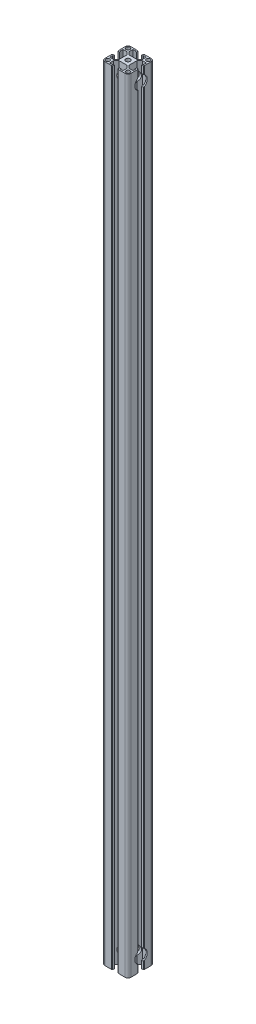
from build123d import *

# Parameters (mm, degrees)
SKETCH16_R          = 3.4
SKETCH16_R_2        = 3
MEMBER_1_DEPTH      = 1203
SKETCH_2_R          = 9.5
CUT_EXTRUDE_1_DEPTH = 1204.830968201


with BuildPart() as part:
    # Sketch16 → Member 1 (new body)
    with BuildSketch(Plane(origin=(0, 0, 0), x_dir=(-1, 0, 0), z_dir=(0, 1, 0))):
        with BuildLine():
            Line((-5.1, 20), (-5.1, 19.5))
            Line((-5.1, 19.5), (-4.1, 19.5))
            Line((-4.1, 19.5), (-4.1, 17))
            Line((-4.1, 17), (-6.1, 17))
            Line((-6.1, 17), (-6.1, 18))
            Line((-6.1, 18), (-10.3, 18))
            Line((-10.3, 18), (-10.3, 12))
            Line((-10.3, 12), (-6, 7.7))
            Line((-6, 7.7), (6, 7.7))
            Line((6, 7.7), (10.3, 12))
            Line((10.3, 12), (10.3, 18))
            Line((10.3, 18), (6.1, 18))
            Line((6.1, 18), (6.1, 17))
            Line((6.1, 17), (4.1, 17))
            Line((4.1, 17), (4.1, 19.5))
            Line((4.1, 19.5), (5.1, 19.5))
            Line((5.1, 19.5), (5.1, 20))
            Line((5.1, 20), (15.5, 20))
            ThreePointArc((15.5, 20), (18.681980515, 18.681980515), (20, 15.5))
            Line((20, 15.5), (20, 5.1))
            Line((20, 5.1), (19.5, 5.1))
            Line((19.5, 5.1), (19.5, 4.1))
            Line((19.5, 4.1), (17, 4.1))
            Line((17, 4.1), (17, 6.1))
            Line((17, 6.1), (18, 6.1))
            Line((18, 6.1), (18, 10.3))
            Line((18, 10.3), (12, 10.3))
            Line((12, 10.3), (7.7, 6))
            Line((7.7, 6), (7.7, -6))
            Line((7.7, -6), (12, -10.3))
            Line((12, -10.3), (18, -10.3))
            Line((18, -10.3), (18, -6.1))
            Line((18, -6.1), (17, -6.1))
            Line((17, -6.1), (17, -4.1))
            Line((17, -4.1), (19.5, -4.1))
            Line((19.5, -4.1), (19.5, -5.1))
            Line((19.5, -5.1), (20, -5.1))
            Line((20, -5.1), (20, -15.5))
            ThreePointArc((20, -15.5), (18.681980515, -18.681980515), (15.5, -20))
            Line((15.5, -20), (5.1, -20))
            Line((5.1, -20), (5.1, -19.5))
            Line((5.1, -19.5), (4.1, -19.5))
            Line((4.1, -19.5), (4.1, -17))
            Line((4.1, -17), (6.1, -17))
            Line((6.1, -17), (6.1, -18))
            Line((6.1, -18), (10.3, -18))
            Line((10.3, -18), (10.3, -12))
            Line((10.3, -12), (6, -7.7))
            Line((6, -7.7), (-6, -7.7))
            Line((-6, -7.7), (-10.3, -12))
            Line((-10.3, -12), (-10.3, -18))
            Line((-10.3, -18), (-6.1, -18))
            Line((-6.1, -18), (-6.1, -17))
            Line((-6.1, -17), (-4.1, -17))
            Line((-4.1, -17), (-4.1, -19.5))
            Line((-4.1, -19.5), (-5.1, -19.5))
            Line((-5.1, -19.5), (-5.1, -20))
            Line((-5.1, -20), (-15.5, -20))
            ThreePointArc((-15.5, -20), (-18.681980515, -18.681980515), (-20, -15.5))
            Line((-20, -15.5), (-20, -5.1))
            Line((-20, -5.1), (-19.5, -5.1))
            Line((-19.5, -5.1), (-19.5, -4.1))
            Line((-19.5, -4.1), (-17, -4.1))
            Line((-17, -4.1), (-17, -6.1))
            Line((-17, -6.1), (-18, -6.1))
            Line((-18, -6.1), (-18, -10.3))
            Line((-18, -10.3), (-12, -10.3))
            Line((-12, -10.3), (-7.7, -6))
            Line((-7.7, -6), (-7.7, 6))
            Line((-7.7, 6), (-12, 10.3))
            Line((-12, 10.3), (-18, 10.3))
            Line((-18, 10.3), (-18, 6.1))
            Line((-18, 6.1), (-17, 6.1))
            Line((-17, 6.1), (-17, 4.1))
            Line((-17, 4.1), (-19.5, 4.1))
            Line((-19.5, 4.1), (-19.5, 5.1))
            Line((-19.5, 5.1), (-20, 5.1))
            Line((-20, 5.1), (-20, 15.5))
            ThreePointArc((-20, 15.5), (-18.681980515, 18.681980515), (-15.5, 20))
            Line((-15.5, 20), (-5.1, 20))
        make_face()
        Circle(SKETCH16_R, mode=Mode.SUBTRACT)
        with Locations((-15.556349186, 15.556349186)):
            Circle(SKETCH16_R_2, mode=Mode.SUBTRACT)
        with Locations((15.556349186, 15.556349186)):
            Circle(SKETCH16_R_2, mode=Mode.SUBTRACT)
        with Locations((15.556349186, -15.556349186)):
            Circle(SKETCH16_R_2, mode=Mode.SUBTRACT)
        with Locations((-15.556349186, -15.556349186)):
            Circle(SKETCH16_R_2, mode=Mode.SUBTRACT)
    extrude(amount=MEMBER_1_DEPTH)

    # 草图2 → 切除-拉伸1 (cut, through all)
    with BuildSketch(Plane.ZY.offset(20)):
        with Locations(Location((0, 1183, 0), (0, 0, 309.166710716))):
            Circle(SKETCH_2_R)
        with Locations(Location((0, 20, 0), (0, 0, 309.166710716))):
            Circle(SKETCH_2_R)
    extrude(amount=-CUT_EXTRUDE_1_DEPTH, mode=Mode.SUBTRACT)


solid = part.part
